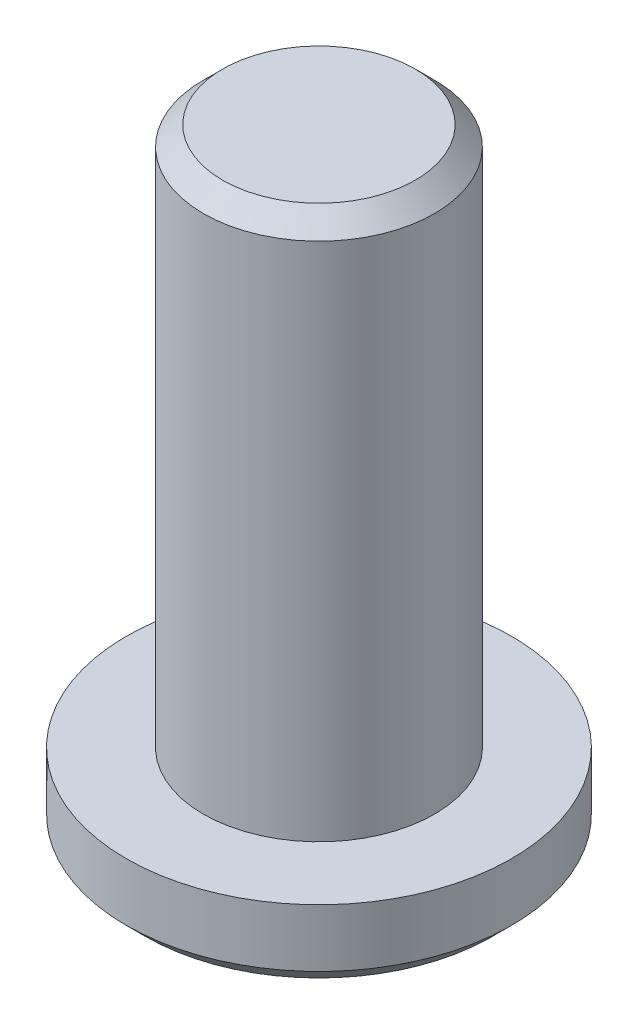
from build123d import *

# Parameters (mm, degrees)
SKETCH1_R           = 5
BOSS_EXTRUDE1_DEPTH = 2
SKETCH2_R           = 3
BOSS_EXTRUDE2_DEPTH = 14
CHAMFER1_SIZE       = 0.5


with BuildPart() as part:
    # Sketch1 → Boss-Extrude1 (new body)
    with BuildSketch(Plane(origin=(0, 0, 0), x_dir=(1, 0, 0), z_dir=(0, 1, 0))):
        with Locations(Location((0, 0, 0), (0, 0, 270))):
            Circle(SKETCH1_R)
    extrude(amount=BOSS_EXTRUDE1_DEPTH)

    # Sketch2 → Boss-Extrude2 (add)
    with BuildSketch(Plane(origin=(0, 2, 0), x_dir=(1, 0, 0), z_dir=(0, 1, 0))):
        with Locations(Location((0, 0, 0), (0, 0, 270))):
            Circle(SKETCH2_R)
    extrude(amount=BOSS_EXTRUDE2_DEPTH)

    # Chamfer1
    chamfer1_edges = [part.edges().sort_by_distance(p)[0] for p in [
        (0, 0, -5),
        (0, 16, -3),
    ]]
    chamfer(chamfer1_edges, length=CHAMFER1_SIZE)


solid = part.part
